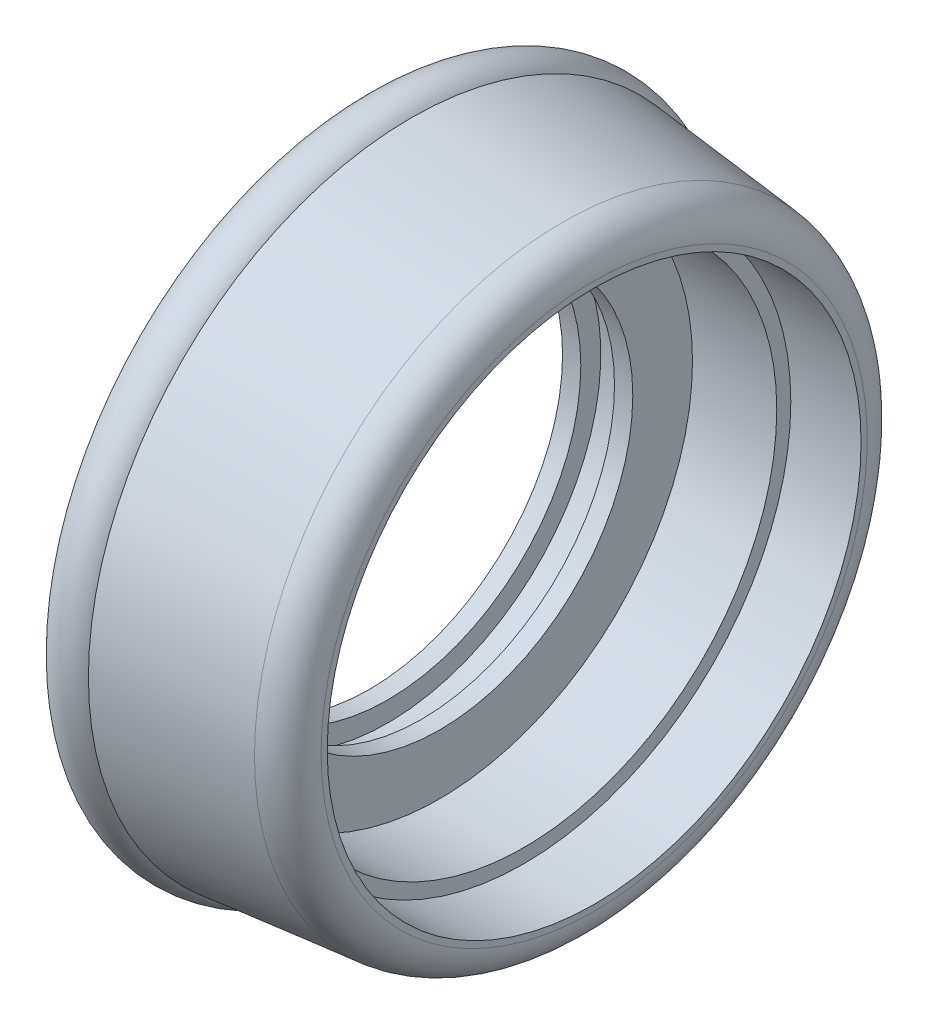
SolidWorks part; units mm, degrees
material "普通碳钢"
ref_plane "Front Plane" through (0, 0, 0) normal (0, 0, 1) x (1, 0, 0)
ref_plane "Top Plane" through (0, 0, 0) normal (0, 1, 0) x (1, 0, 0)
ref_plane "Right Plane" through (0, 0, 0) normal (1, 0, 0) x (0, 0, -1)
sketch "Sketch1" plane through (0, 0, 0) normal (0, 0, 1) x (1, 0, 0)
  line L0 (-44.6819, 0) -> (116.6227, 0) construction
  line L1 (0, 27.5) -> (0, 46)
  line L2 (0, 0) -> (0, 27.5) construction
  line L3 (32, 38.8751) -> (32, 38)
  line L4 (27.4975, 43.8502) -> (6, 46)
  line L5 (22, 38) -> (22, 36)
  line L6 (22, 38) -> (32, 38)
  line L7 (22, 36) -> (10, 36)
  line L8 (10, 36) -> (10, 27.5)
  line L9 (10, 27.5) -> (7.4, 27.5)
  line L10 (2.6, 30.35) -> (7.4, 30.35)
  line L11 (2.6, 30.35) -> (2.6, 27.5)
  line L12 (7.4, 30.35) -> (7.4, 27.5)
  line L14 (2.6, 27.5) -> (0, 27.5)
  arc A0 (6, 46) -> (0, 46) centre (3, 43.3542) ccw
  arc A1 (27.4975, 43.8502) -> (32, 38.8751) centre (27, 38.8751) cw
  point P13 (32, 43.4)
  dimension "D4" = 8
  dimension "D7" = 5
  dimension "D2" = 46
  dimension "D3" = 46
  dimension "D5" = 32
  dimension "D6" = 6
  dimension "D8" = 10
  dimension "D9" = 38
  dimension "D10" = 36
  dimension "D11" = 12
  dimension "D12" = 27.5
  dimension "D13" = 60.7
  dimension "D14" = 2.6
  dimension "D15" = 4.8
  dimension "D16" = 43.4
revolve "Revolve1" add sketch "Sketch1" angle 360 about L0
